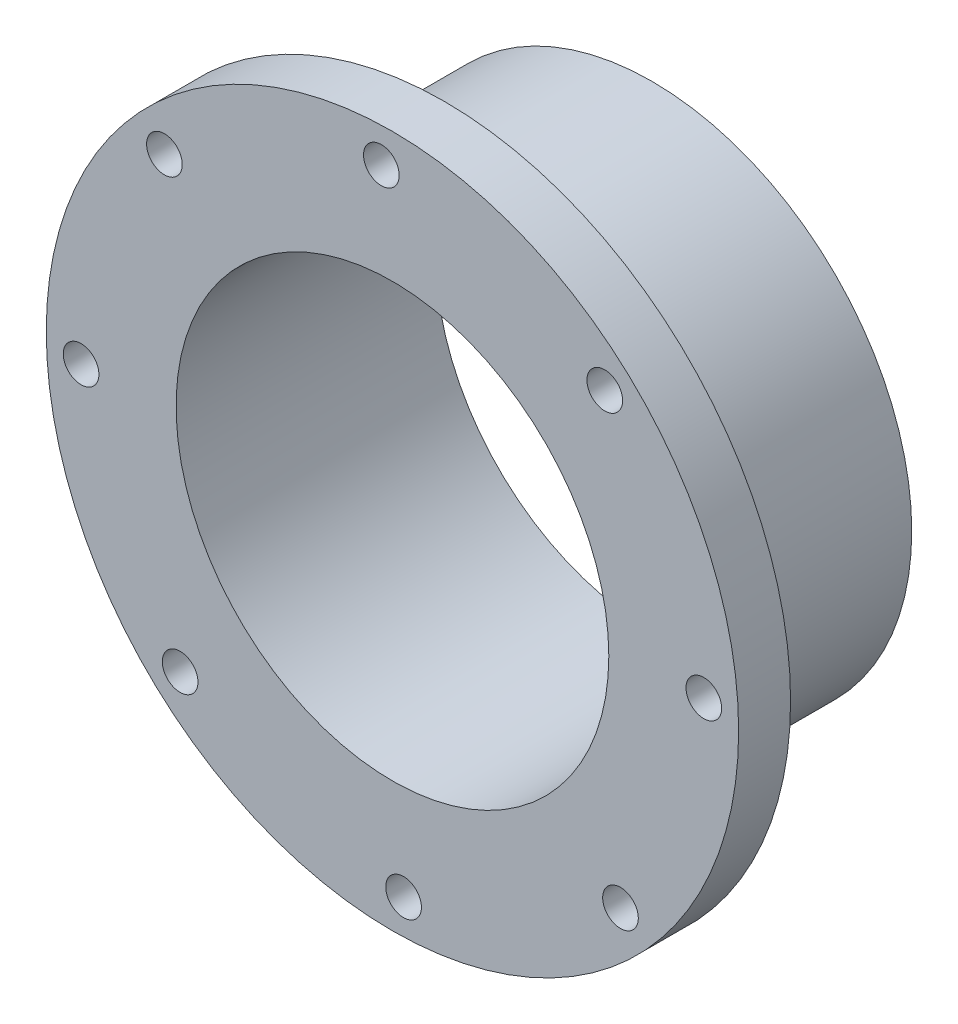
from build123d import *

# Parameters (mm, degrees)
SKETCH1_R           = 15
SKETCH1_R_2         = 12.5
BOSS_EXTRUDE1_DEPTH = 5
SKETCH2_R           = 15
SKETCH2_R_2         = 12.5
BOSS_EXTRUDE2_DEPTH = 10
SKETCH3_R           = 20
SKETCH3_R_2         = 14.885772681
BOSS_EXTRUDE5_DEPTH = 3
SKETCH6_R           = 1.03
CUT_EXTRUDE9_DEPTH  = 10


with BuildPart() as part:
    # Sketch1 → Boss-Extrude1 (new body)
    with BuildSketch(Plane.XY):
        Circle(SKETCH1_R)
        Circle(SKETCH1_R_2, mode=Mode.SUBTRACT)
    extrude(amount=BOSS_EXTRUDE1_DEPTH)

    # Sketch2 → Boss-Extrude2 (add)
    with BuildSketch(Plane.XY.offset(5)):
        Circle(SKETCH2_R)
        Circle(SKETCH2_R_2, mode=Mode.SUBTRACT)
    extrude(amount=BOSS_EXTRUDE2_DEPTH)

    # Sketch3 → Boss-Extrude5 (add)
    with BuildSketch(Plane.XY.offset(12)):
        Circle(SKETCH3_R)
        Circle(SKETCH3_R_2, mode=Mode.SUBTRACT)
    extrude(amount=BOSS_EXTRUDE5_DEPTH)

    # Sketch6 → Cut-Extrude9 (cut)
    with BuildSketch(Plane.XY.offset(15)):
        with Locations((17.988559183, 0.641668533)):
            Circle(SKETCH6_R)
        with Locations((13.173560353, -12.266104012)):
            Circle(SKETCH6_R)
        with Locations((0.641668533, -17.988559183)):
            Circle(SKETCH6_R)
        with Locations((-12.266104012, -13.173560353)):
            Circle(SKETCH6_R)
        with Locations((-17.988559183, -0.641668533)):
            Circle(SKETCH6_R)
        with Locations((-13.173560353, 12.266104012)):
            Circle(SKETCH6_R)
        with Locations((-0.641668533, 17.988559183)):
            Circle(SKETCH6_R)
        with Locations((12.266104012, 13.173560353)):
            Circle(SKETCH6_R)
    extrude(amount=-CUT_EXTRUDE9_DEPTH, mode=Mode.SUBTRACT)


solid = part.part
